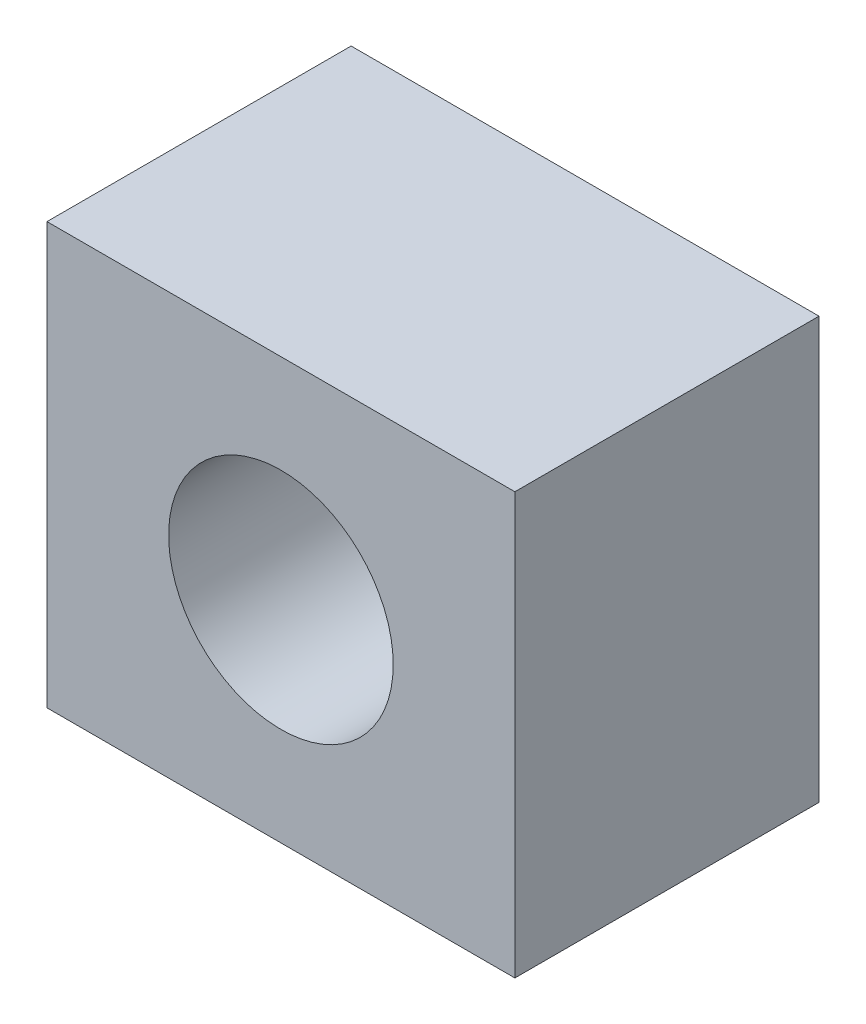
from build123d import *

# Parameters (mm, degrees)
SKETCH1_W           = 100
SKETCH1_H           = 90
SKETCH1_R           = 24
BOSS_EXTRUDE1_DEPTH = 65


with BuildPart() as part:
    # Sketch1 → Boss-Extrude1 (new body)
    with BuildSketch(Plane.XY):
        with Locations((50, 45)):
            Rectangle(SKETCH1_W, SKETCH1_H)
        with Locations((50, 45)):
            Circle(SKETCH1_R, mode=Mode.SUBTRACT)
    extrude(amount=BOSS_EXTRUDE1_DEPTH)


solid = part.part
